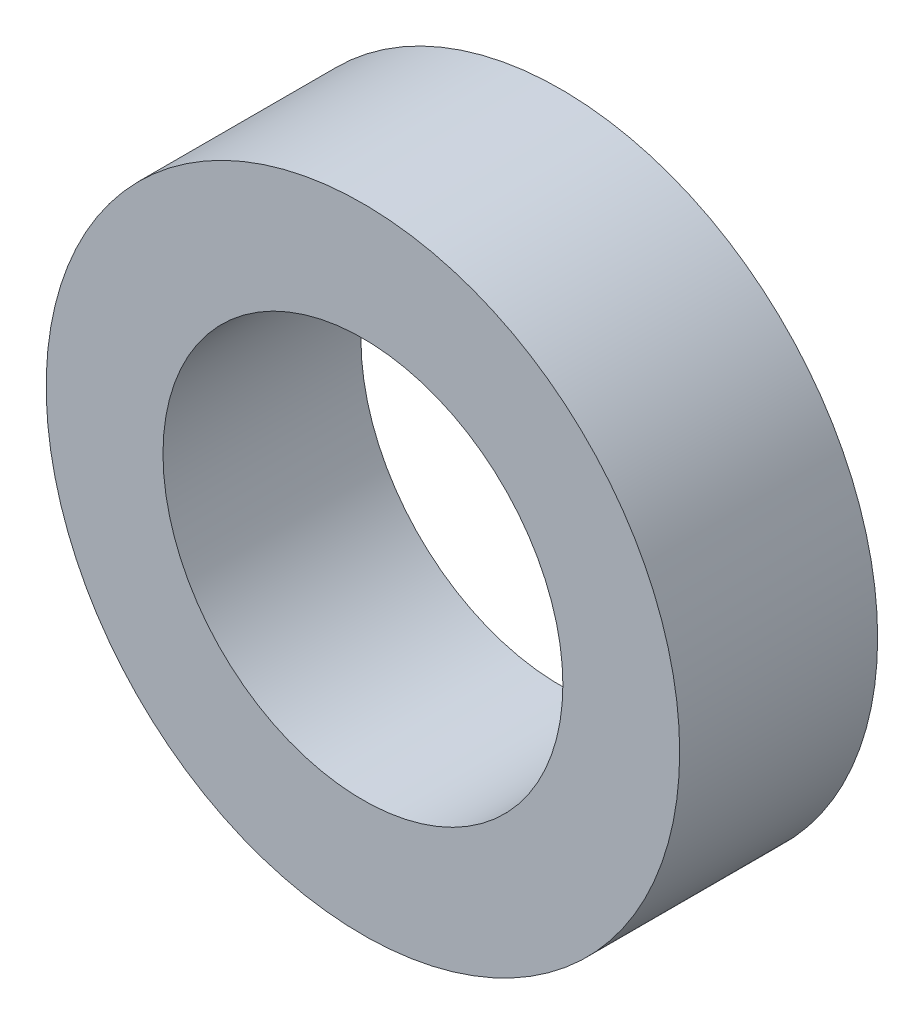
from build123d import *

# Parameters (mm, degrees)
SKETCH_1_R      = 16
SKETCH_1_R_2    = 10.1
EXTRUDE_1_DEPTH = 5


with BuildPart() as part:
    # 草图1 → 凸台-拉伸1 (new, symmetric)
    with BuildSketch(Plane.XY):
        Circle(SKETCH_1_R)
        Circle(SKETCH_1_R_2, mode=Mode.SUBTRACT)
    extrude(amount=EXTRUDE_1_DEPTH, both=True)


solid = part.part
